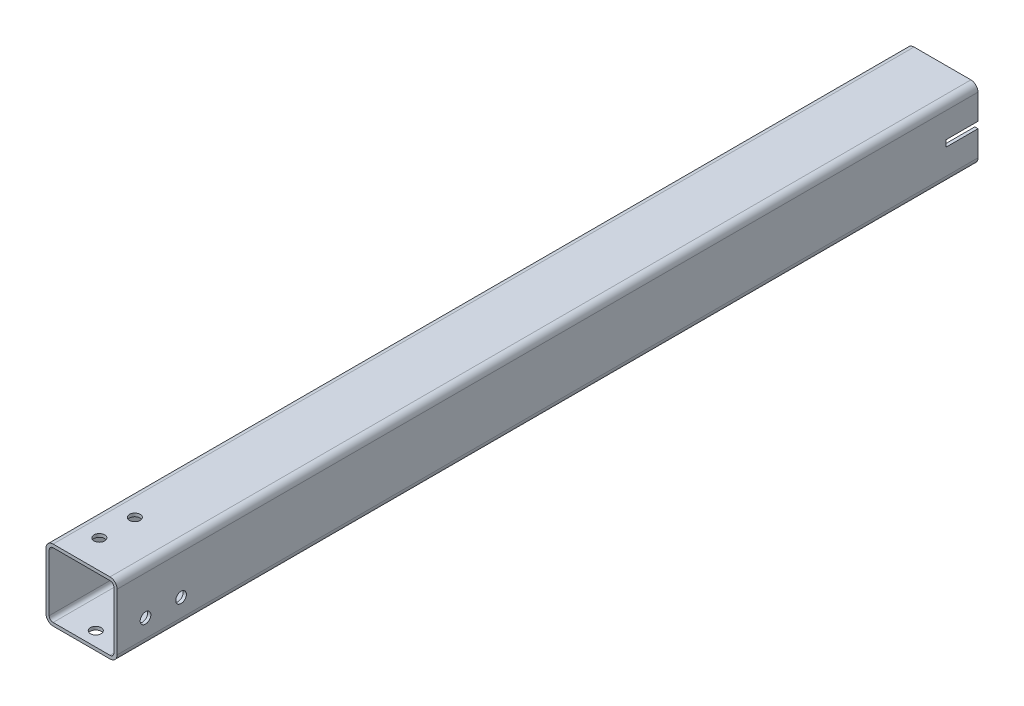
SolidWorks part; units mm, degrees
material "STKR400"
ref_plane "Plane1" through (0, 0, 0) normal (0, 0, 1) x (1, 0, 0)
ref_plane "Plane2" through (0, 0, 0) normal (0, 1, 0) x (1, 0, 0)
ref_plane "Plane3" through (0, 0, 0) normal (1, 0, 0) x (0, 0, -1)
sketch "Sketch1" plane through (0, 0, 0) normal (0, 0, 1) x (1, 0, 0)
  line L0 (-40, -45.5) -> (40, -45.5)
  line L1 (-45.5, -40) -> (-45.5, 40)
  line L2 (40, 45.5) -> (-40, 45.5)
  line L3 (45.5, 40) -> (45.5, -40)
  line L4 (-40, -50) -> (40, -50)
  line L5 (-50, -40) -> (-50, 40)
  line L6 (40, 50) -> (-40, 50)
  line L7 (50, 40) -> (50, -40)
  arc A0 (50, 40) -> (40, 50) centre (40, 40) ccw
  arc A1 (40, -50) -> (50, -40) centre (40, -40) ccw
  arc A2 (-50, -40) -> (-40, -50) centre (-40, -40) ccw
  arc A3 (-40, 50) -> (-50, 40) centre (-40, 40) ccw
  arc A4 (-40, 45.5) -> (-45.5, 40) centre (-40, 40) ccw
  arc A5 (45.5, 40) -> (40, 45.5) centre (40, 40) ccw
  arc A6 (40, -45.5) -> (45.5, -40) centre (40, -40) ccw
  arc A7 (-45.5, -40) -> (-40, -45.5) centre (-40, -40) ccw
  point P0 (-50, 0)
  point P1 (50, 0)
  point P2 (0, 50)
  point P3 (0, -50)
  point P4 (0, 0)
  point P5 (-50, -50)
  point P6 (50, -50)
  point P7 (50, 50)
  point P8 (-50, 50)
extrude "Boss-Extrude1" add sketch "Sketch1" along normal blind 1211
sketch "草图1" plane through (50, 0, 0) normal (1, 0, 0) x (0, 0, -1)
  line L6 (-1211, -40) -> (-1211, 40) construction
  line L7 (-1211, 50) -> (0, 50) construction
  circle A0 centre (-1171, -15) radius 7.5
  circle A1 centre (-1121, -15) radius 7.5
  dimension "D1" = 15
  dimension "D2" = 40
  dimension "D3" = 50
  dimension "D4" = 65
extrude "Cut-Extrude1" cut sketch "草图1" against normal up to next
sketch "Sketch2" plane through (0, -50, 0) normal (0, -1, 0) x (1, 0, 0)
  line L0 (-40, 1211) -> (40, 1211) construction
  circle A0 centre (0, 1191) radius 7.5
  circle A1 centre (0, 1121) radius 7.5
  circle A2 centre (0, 20) radius 7.5
  dimension "D1" = 15
  dimension "D2" = 20
  dimension "D3" = 70
  dimension "D4" = 20
extrude "Cut-Extrude2" cut sketch "Sketch2" against normal up to next
sketch "Sketch3" plane through (0, 50, 0) normal (0, 1, 0) x (1, 0, 0)
  line L0 (40, -1211) -> (-40, -1211) construction
  line L1 (50, -1211) -> (50, 0) construction
  circle A0 centre (-15, -1171) radius 7.5
  circle A1 centre (-15, -1121) radius 7.5
  dimension "D1" = 40
  dimension "D2" = 50
  dimension "D3" = 65
  dimension "D4" = 15
extrude "Cut-Extrude3" cut sketch "Sketch3" against normal up to next
sketch "Sketch4" plane through (50, 0, 0) normal (1, 0, 0) x (0, 0, -1)
  line L0 (0, -40) -> (0, 40) construction
  line L1 (0, -4.5) -> (-45, -4.5)
  line L2 (0, -4.5) -> (0, 4.5)
  line L3 (0, 4.5) -> (-45, 4.5)
  line L4 (-45, -4.5) -> (-45, 4.5)
  line L5 (-1211, -50) -> (0, -50) construction
  dimension "D1" = 9
  dimension "D2" = 45.5
  dimension "D3" = 45
extrude "Cut-Extrude4" cut sketch "Sketch4" against normal through all
